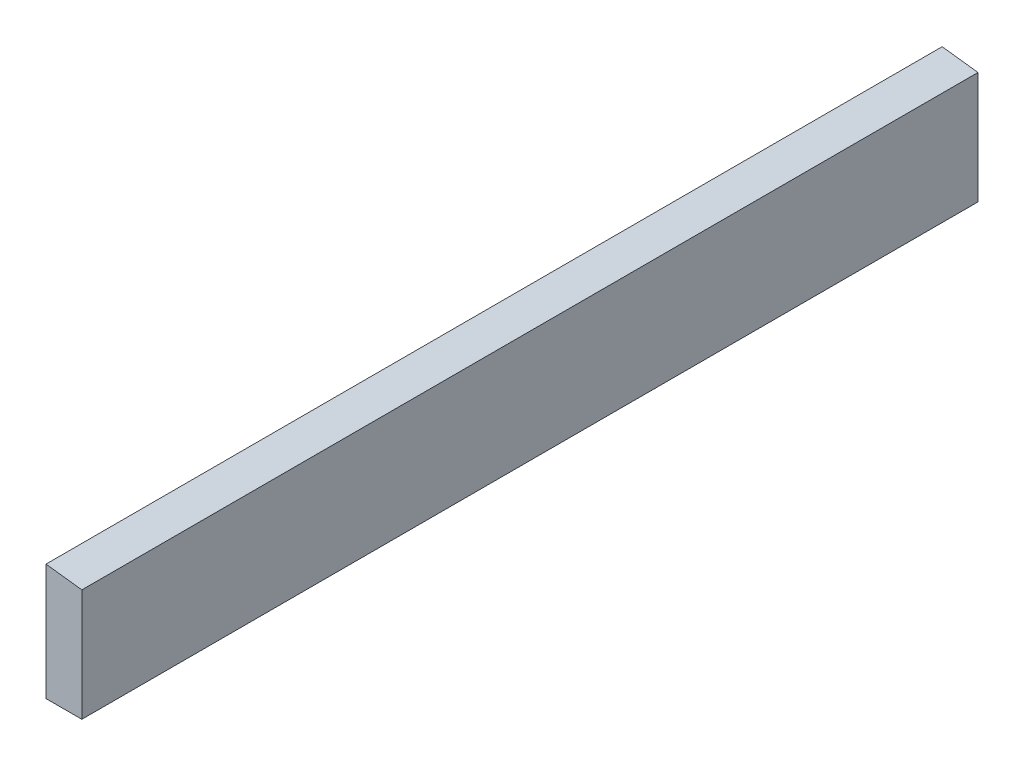
SolidWorks part; units mm, degrees
material "Plain Carbon Steel"
ref_plane "Front Plane" through (0, 0, 0) normal (0, 0, 1) x (1, 0, 0)
ref_plane "Top Plane" through (0, 0, 0) normal (0, 1, 0) x (1, 0, 0)
ref_plane "Right Plane" through (0, 0, 0) normal (1, 0, 0) x (0, 0, -1)
sketch "Sketch1" plane through (0, 0, 0) normal (0, 0, 1) x (1, 0, 0)
  line L0 (0, 0) -> (0, 32.5)
  line L1 (0, 0) -> (10, 0)
  line L2 (10, 0) -> (10, 31.2722)
  line L3 (10, 31.2722) -> (0, 32.5)
  dimension "D1" = 32.5
  dimension "D2" = 10
  dimension "D3" = 83
extrude "Boss-Extrude1" add sketch "Sketch1" along normal blind 250
